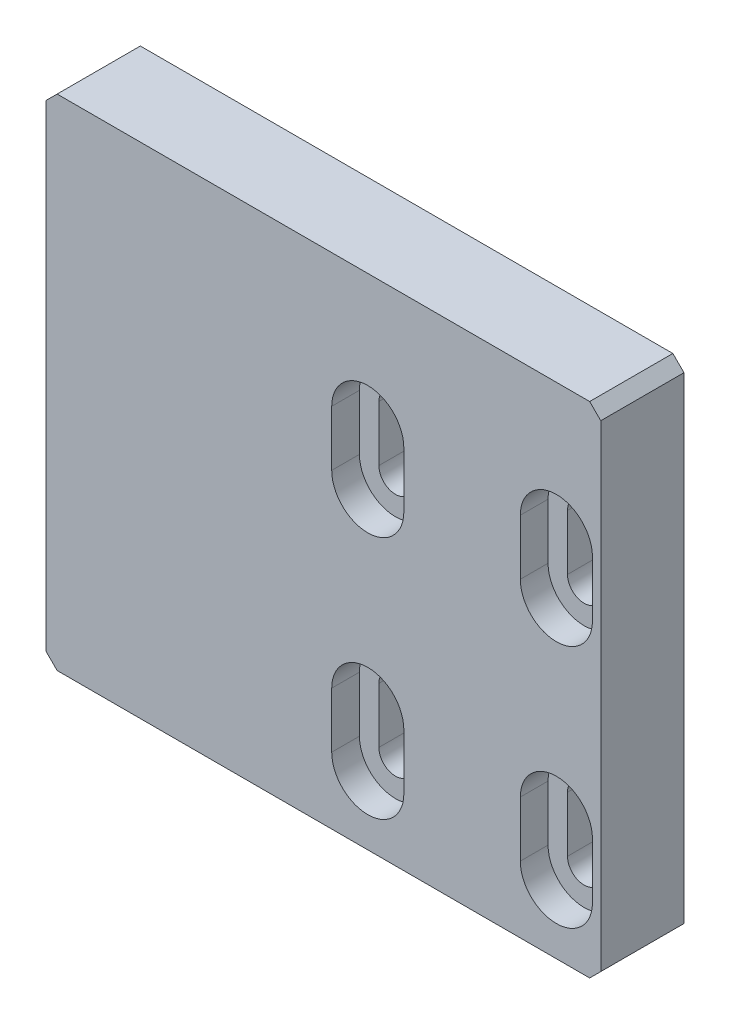
SolidWorks part; units mm, degrees
material "A6061"
ref_plane "前视基准面" through (0, 0, 0) normal (0, 0, 1) x (1, 0, 0)
ref_plane "上视基准面" through (0, 0, 0) normal (0, 1, 0) x (1, 0, 0)
ref_plane "右视基准面" through (0, 0, 0) normal (1, 0, 0) x (0, 0, -1)
sketch "草图1" plane through (0, 0, 0) normal (0, 0, 1) x (1, 0, 0)
  line L1 (-50, -45) -> (50, -45)
  line L2 (-50, -45) -> (-50, 45)
  line L3 (-50, 45) -> (50, 45)
  line L4 (50, -45) -> (50, 45)
  line L5 (-50, -45) -> (50, 45) construction
  line L6 (-50, 45) -> (50, -45) construction
  point P0 (0, 0)
  dimension "D1" = 100
  dimension "D2" = 90
extrude "凸台-拉伸1" add sketch "草图1" against normal mid plane 15
hole_wizard "M6 螺纹孔1" positions "草图3" profile "草图2" tap size "M6" standard "GB"
sketch "草图3" plane through (-50, 0, 0) normal (-1, 0, 0) x (0, 0, 1)
  line L0 (-7.5, 45) -> (7.5, 45) construction
  line L1 (0, 45) -> (0, 35) construction
  line L2 (0, 35) -> (0, 0) construction
  line L3 (0, 0) -> (0, -35) construction
  point P0 (0, 35)
  point P8 (0, 0)
  point P11 (0, -35)
  dimension "D1" = 10
sketch "草图2" plane through (-50, 35, 0) normal (0, 1, 0) x (0, 0, 1)
  line L0 (0, 0) -> (0, 16.5022)
  line L1 (0, 16.5022) -> (2.5, 15)
  line L2 (2.5, 15) -> (2.5, 0)
  line L5 (2.5, 0) -> (0, 0)
  line L10 (0, 16.5022) -> (-2.5, 15) construction
  line L11 (0, -6.35) -> (0, 107.95) construction
  dimension "螺纹孔钻头直径" = 5
  dimension "螺纹孔钻头深度" = 15
  dimension "导头角度" = 118
cosmetic thread "孔螺蚊线1" parameters "D1"=12, "D2"=6
cosmetic thread "孔螺蚊线2" parameters "D1"=12, "D2"=6
cosmetic thread "孔螺蚊线3" parameters "D1"=12, "D2"=6
sketch "草图4" plane through (0, 0, 7.5) normal (0, 0, 1) x (1, 0, 0)
  line L0 (8, -23) -> (8, -33) construction
  line L1 (14.5, -23) -> (14.5, -33)
  line L2 (1.5, -23) -> (1.5, -33)
  line L3 (-50, -45) -> (50, -45) construction
  line L4 (50, -45) -> (50, 45) construction
  arc A0 (14.5, -23) -> (1.5, -23) centre (8, -23) ccw
  arc A1 (1.5, -33) -> (14.5, -33) centre (8, -33) ccw
  point P2 (8, -28)
  dimension "D2" = 6.5
  dimension "D3" = 12
  dimension "D4" = 42
  dimension "D1" = 10
extrude "切除-拉伸1" cut sketch "草图4" against normal blind 5
sketch "草图5" plane through (0, 0, 2.5) normal (0, 0, 1) x (1, 0, 0)
  line L4 (5, -23) -> (5, -33)
  line L5 (11, -33) -> (11, -23)
  line L6 (5, -23) -> (5, -33)
  line L7 (11, -33) -> (11, -23)
  arc A4 (11, -23) -> (5, -23) centre (8, -23) ccw
  arc A5 (5, -33) -> (11, -33) centre (8, -33) ccw
  arc A6 (11, -23) -> (5, -23) centre (8, -23) ccw
  arc A7 (5, -33) -> (11, -33) centre (8, -33) ccw
  dimension "D2" = 3
  dimension "D1" = 3.5
extrude "切除-拉伸2" cut sketch "草图5" against normal through all
pattern_linear "阵列(线性)1" count 2 spacing 34 along (1, 0, 0) count 2 spacing 44 along (0, 1, 0) of "切除-拉伸1", "切除-拉伸2"
chamfer "倒角1" distance 2 angle 45 4 edges at (-50, -45, 0) (50, -45, 0) (50, 45, 0) (-50, 45, 0)
